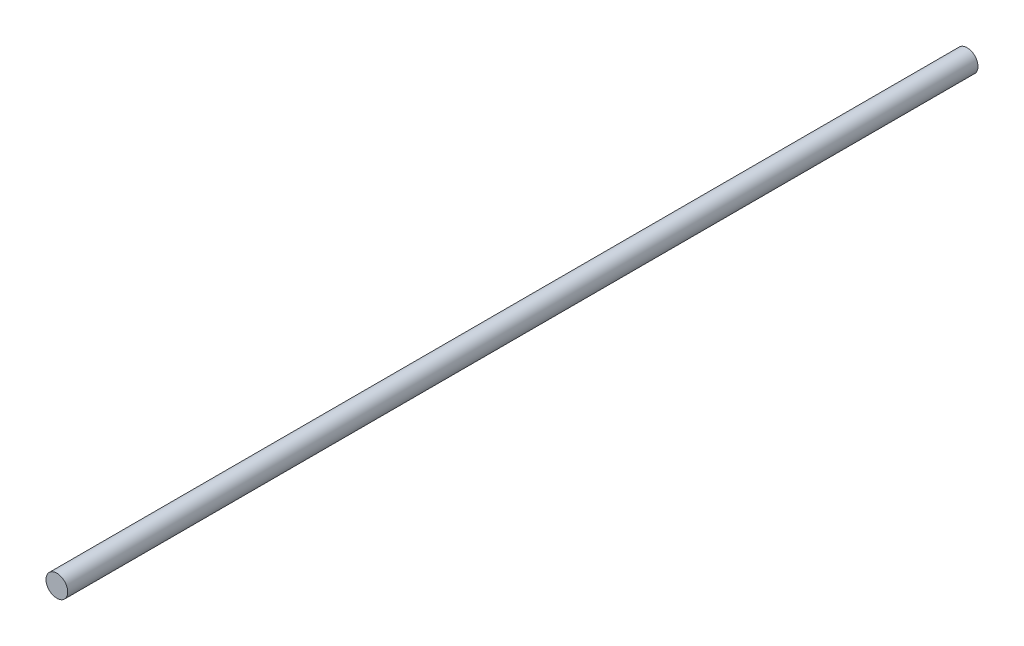
from build123d import *

# Parameters (mm, degrees)
SKETCH1_R           = 8
BOSS_EXTRUDE1_DEPTH = 669


with BuildPart() as part:
    # Sketch1 → Boss-Extrude1 (new body)
    with BuildSketch(Plane.XY):
        Circle(SKETCH1_R)
    extrude(amount=BOSS_EXTRUDE1_DEPTH)


solid = part.part
